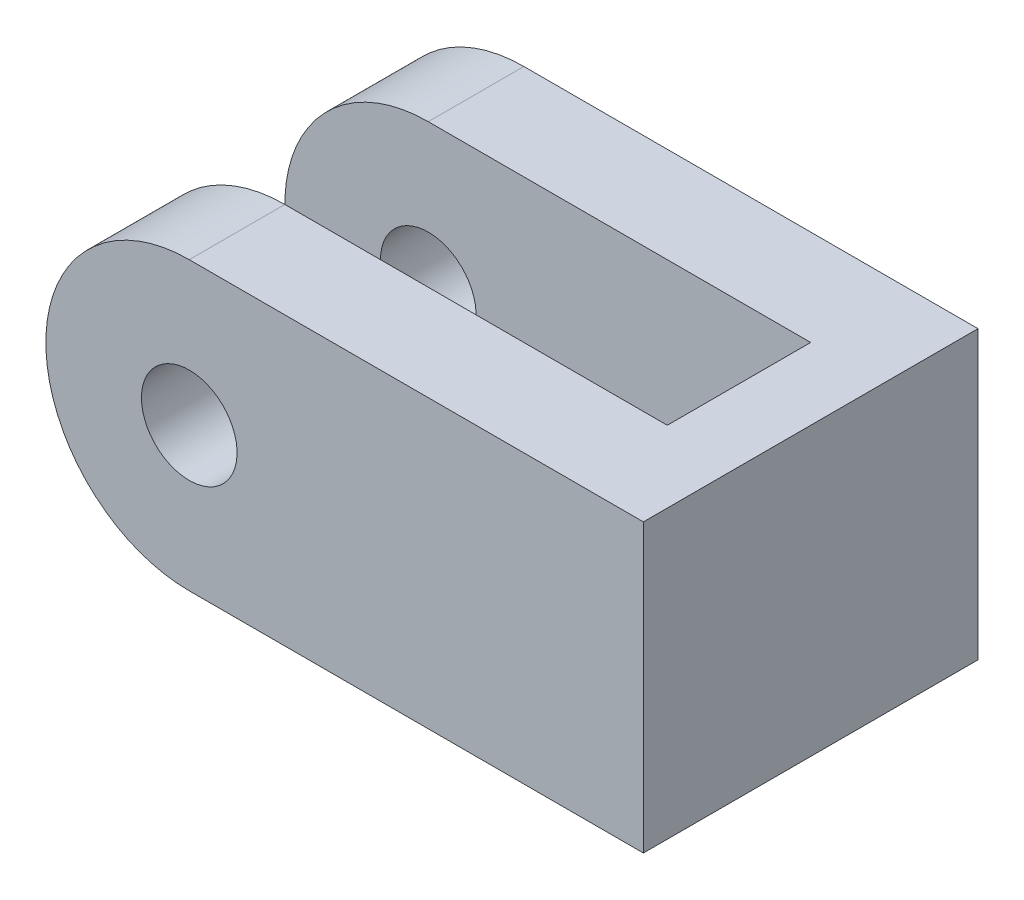
SolidWorks part; units mm, degrees
ref_plane "Front Plane" through (0, 0, 0) normal (0, 0, 1) x (1, 0, 0)
ref_plane "Top Plane" through (0, 0, 0) normal (0, 1, 0) x (1, 0, 0)
ref_plane "Right Plane" through (0, 0, 0) normal (1, 0, 0) x (0, 0, -1)
sketch "Sketch1" plane through (0, 0, 0) normal (0, 0, 1) x (1, 0, 0)
  line L1 (-40, 30) -> (40, 30)
  line L3 (-40, -30) -> (40, -30)
  line L4 (40, 30) -> (40, -30)
  line L5 (-40, 30) -> (40, -30) construction
  line L6 (-40, -30) -> (40, 30) construction
  arc A0 (-40, 30) -> (-40, -30) centre (-40, 0) ccw
  point P0 (0, 0)
  dimension "D1" = 80
  dimension "D2" = 60
extrude "Boss-Extrude1" add sketch "Sketch1" along normal blind 20
sketch "Sketch2" plane through (0, 0, 0) normal (0, 0, -1) x (-1, 0, 0)
  circle A0 centre (40, 0) radius 10
  dimension "D1" = 20
extrude "Cut-Extrude1" cut sketch "Sketch2" against normal through all
sketch "Sketch3" plane through (40, 0, 0) normal (1, 0, 0) x (0, 0, -1)
  line L0 (-20, -30) -> (-20, 30)
  line L1 (-20, -30) -> (15, -30)
  line L2 (-20, 30) -> (15, 30)
  line L3 (15, -30) -> (15, 30)
  dimension "D1" = 35
extrude "Boss-Extrude5" add sketch "Sketch3" along normal blind 15
mirror "Mirror1" about plane through (55, -30, -15) normal (0, 0, 1) of bodies 103
